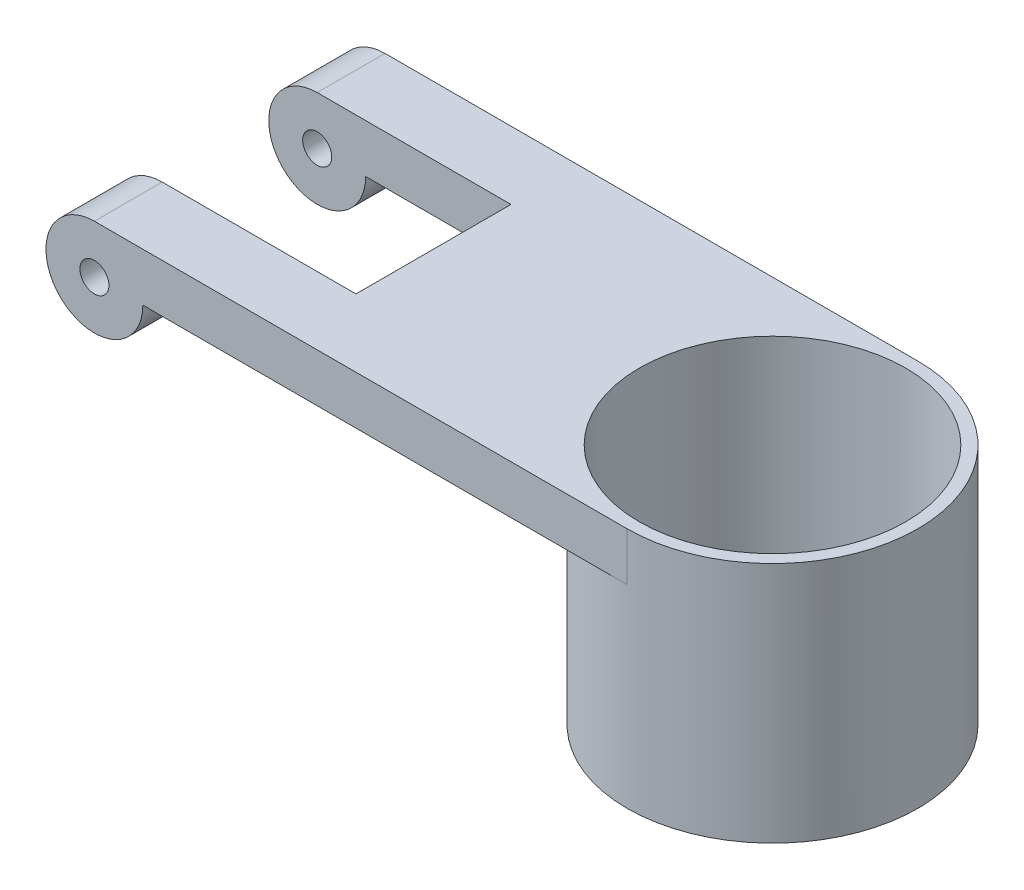
SolidWorks part; units mm, degrees
ref_plane "Front Plane" through (0, 0, 0) normal (0, 0, 1) x (1, 0, 0)
ref_plane "Top Plane" through (0, 0, 0) normal (0, 1, 0) x (1, 0, 0)
ref_plane "Right Plane" through (0, 0, 0) normal (1, 0, 0) x (0, 0, -1)
sketch "Sketch1" plane through (0, 0, 0) normal (0, 0, 1) x (1, 0, 0)
  circle A0 centre (0, 0) radius 10
  circle A1 centre (0, 0) radius 3
  dimension "D1" = 20
  dimension "D2" = 6
extrude "Boss-Extrude1" add sketch "Sketch1" along normal blind 60
sketch "Sketch3" plane through (0, 0, 60) normal (0, 0, 1) x (1, 0, 0)
  line L0 (0, 10) -> (110, 10)
  line L1 (10, 0) -> (110, 0)
  line L2 (110, 10) -> (110, 0)
  circle A0 centre (0, 0) radius 10 construction
  arc A1 (10, 0) -> (0, 10) centre (0, 0) ccw
  dimension "D1" = 10
  dimension "D2" = 100
extrude "Boss-Extrude2" add sketch "Sketch3" against normal up to surface (60 mm away) up to face at (10, 0, 0)
sketch "Sketch4" plane through (0, 10, 0) normal (0, 1, 0) x (1, 0, 0)
  line L0 (110, -30) -> (-10, -30) construction
  line L1 (110, 0) -> (110, -60) construction
  line L2 (-10, 0) -> (-10, -60) construction
  line L4 (-57.3309, -14) -> (40, -14)
  line L5 (-57.3309, -14) -> (-57.3309, -46)
  line L6 (-57.3309, -46) -> (40, -46)
  line L7 (40, -14) -> (40, -46)
  line L8 (-57.3309, -14) -> (40, -46) construction
  line L9 (-57.3309, -46) -> (40, -14) construction
  point P6 (-8.6654, -30)
  dimension "D1" = 32
  dimension "D2" = 50
extrude "Cut-Extrude1" cut sketch "Sketch4" against normal through all both and the other way through all
sketch "Sketch5" plane through (0, 10, 0) normal (0, 1, 0) x (1, 0, 0)
  line L0 (110, 0) -> (110, -60) construction
  circle A0 centre (110, -30) radius 30
  circle A1 centre (110, -30) radius 27.5
  dimension "D1" = 55
extrude "Boss-Extrude3" add sketch "Sketch5" against normal blind 50
sketch "Sketch6" plane through (0, 10, 0) normal (0, 1, 0) x (1, 0, 0)
  circle A0 centre (110, -30) radius 27.5
extrude "Cut-Extrude2" cut sketch "Sketch6" against normal through all both and the other way through all
